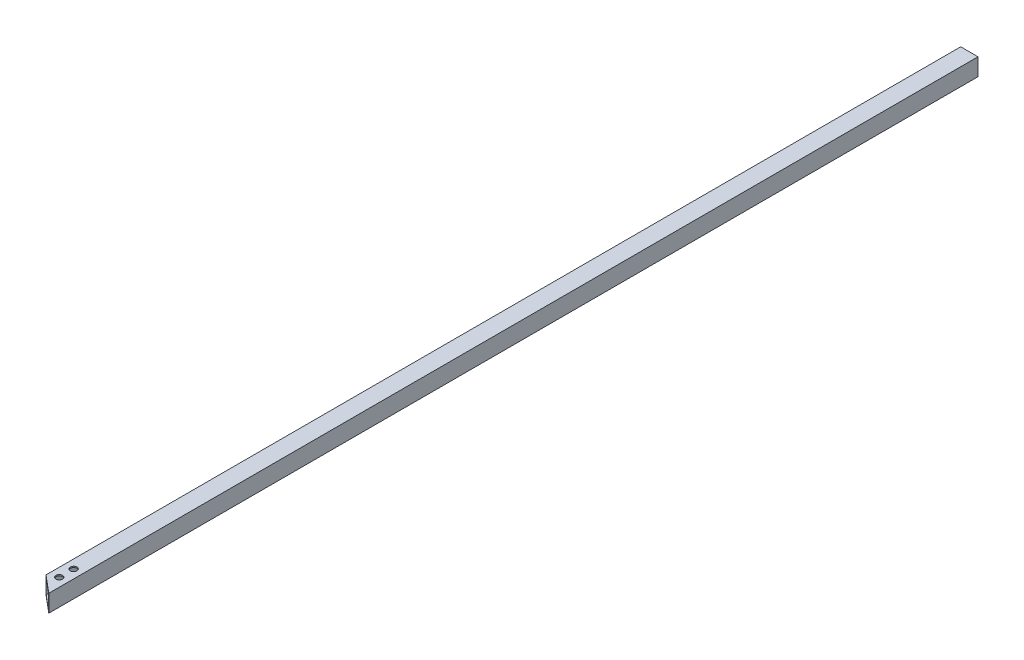
SolidWorks part; units mm, degrees
ref_plane "前视基准面" through (0, 0, 0) normal (0, 0, 1) x (1, 0, 0)
ref_plane "上视基准面" through (0, 0, 0) normal (0, 1, 0) x (1, 0, 0)
ref_plane "右视基准面" through (0, 0, 0) normal (1, 0, 0) x (0, 0, -1)
sketch "草图1" plane through (0, 0, 0) normal (0, 0, 1) x (1, 0, 0)
  line L0 (13, 13) -> (-13, 13)
  line L1 (15, -15) -> (-15, -15)
  line L2 (15, -15) -> (15, 15)
  line L3 (15, 15) -> (-15, 15)
  line L4 (-15, -15) -> (-15, 15)
  line L5 (15, -15) -> (-15, 15) construction
  line L6 (15, 15) -> (-15, -15) construction
  line L7 (-13, -13) -> (-13, 13)
  line L8 (13, -13) -> (-13, -13)
  line L9 (13, -13) -> (13, 13)
  point P0 (0, 0)
  dimension "D1" = 30
  dimension "D2" = 2
extrude "凸台-拉伸1" add sketch "草图1" along normal mid plane 1667
sketch "草图2" plane through (0, 0, -833.5) normal (0, 0, -1) x (-1, 0, 0)
  circle A0 centre (0, 0) radius 6.2521
sketch "草图3" plane through (0, 15, 0) normal (0, 1, 0) x (1, 0, 0)
  line L0 (15, -778.5) -> (-15, -753.327)
  line L1 (15, -833.5) -> (15, 833.5) construction
  line L2 (-15, -833.5) -> (-15, 833.5) construction
  line L7 (15, 833.5) -> (-15, 833.5)
  line L8 (-15, 833.5) -> (-15, -833.5)
  line L9 (-15, -833.5) -> (15, -833.5)
  line L10 (15, -833.5) -> (15, 833.5)
  line L11 (15, 833.5) -> (-15, 833.5)
  line L12 (-15, 833.5) -> (-15, -833.5)
  line L13 (-15, -833.5) -> (15, -833.5)
  line L14 (15, -833.5) -> (15, 833.5)
  line M7 (-15, 833.5) -> (-15, -833.5)
  line M8 (-15, -833.5) -> (15, -833.5)
  line M9 (15, -833.5) -> (15, 833.5)
  dimension "D1" = 0
  dimension "D2" = 40
  dimension "D3" = 55
extrude "切除-拉伸1" cut sketch "草图3" against normal mid plane 70 contours L0 M9 M7 M8
sketch "草图4" plane through (0, -15, 0) normal (0, -1, 0) x (1, 0, 0)
  line L0 (0, 765.9135) -> (0, 745.4135) construction
  line L2 (15, 778.5) -> (-15, 753.327) construction
  line L3 (0, 745.4135) -> (0, 720.4135) construction
  circle A4 centre (0, 745.4135) radius 5.75
  circle A5 centre (0, 720.4135) radius 5.75
  dimension "D1" = 25
  dimension "D3" = 11.5
  dimension "D2" = 20.5
extrude "切除-拉伸2" cut sketch "草图4" against normal blind 163
